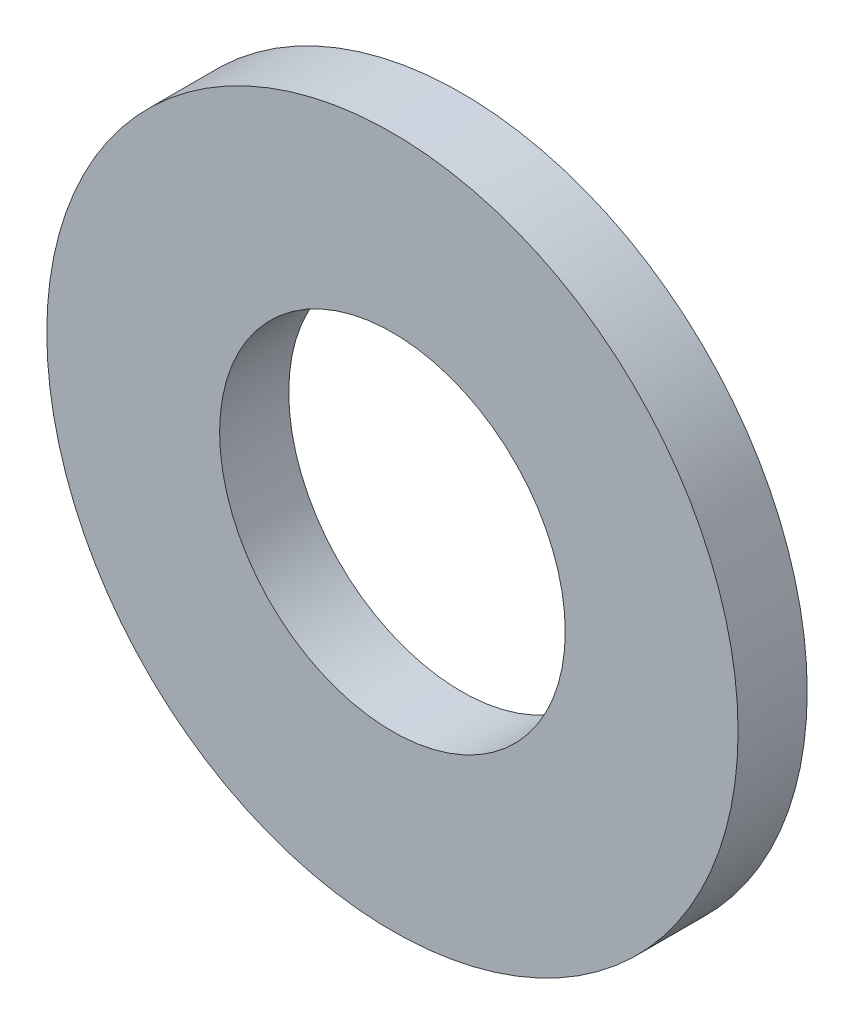
SolidWorks part; units mm, degrees
ref_plane "Front Plane" through (0, 0, 0) normal (0, 0, 1) x (1, 0, 0)
ref_plane "Top Plane" through (0, 0, 0) normal (0, 1, 0) x (1, 0, 0)
ref_plane "Right Plane" through (0, 0, 0) normal (1, 0, 0) x (0, 0, -1)
sketch "Sketch2" plane through (0, 0, 0) normal (0, 0, 1) x (1, 0, 0)
  circle A0 centre (-70, 25) radius 25
extrude "Boss-Extrude1" add sketch "Sketch2" along normal mid plane 5 contours A0
sketch "Sketch3" plane through (0, 0, -2.5) normal (0, 0, -1) x (-1, 0, 0)
  circle A0 centre (70, 25) radius 12.5
extrude "Cut-Extrude1" cut sketch "Sketch3" against normal through all
